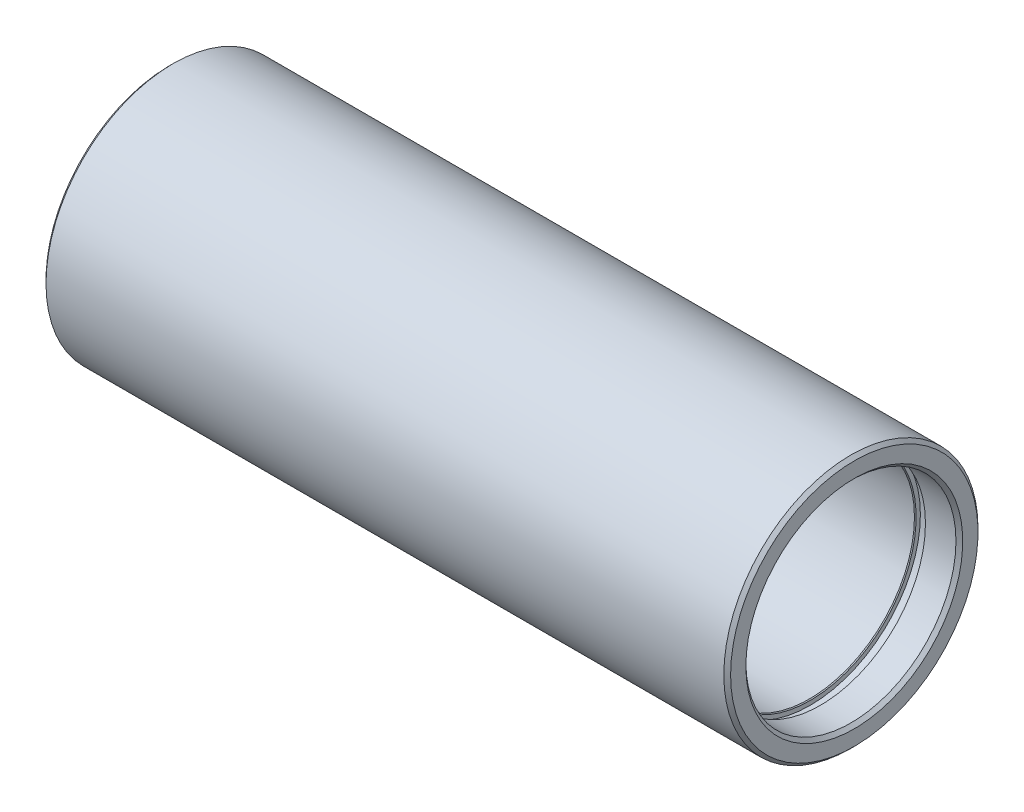
SolidWorks part; units mm, degrees
ref_plane "前视基准面" through (0, 0, 0) normal (0, 0, 1) x (1, 0, 0)
ref_plane "上视基准面" through (0, 0, 0) normal (0, 1, 0) x (1, 0, 0)
ref_plane "右视基准面" through (0, 0, 0) normal (1, 0, 0) x (0, 0, -1)
sketch "草图1" plane through (0, 0, 0) normal (0, 0, 1) x (1, 0, 0)
  line L0 (0, 0) -> (96.9258, 0) construction
  line L1 (-4.1244, 31) -> (5.8756, 31)
  line L2 (5.8756, 31) -> (5.8756, 32.5)
  line L3 (5.8756, 32.5) -> (8.8756, 32.5)
  line L4 (8.8756, 32.5) -> (8.8756, 31)
  line L5 (8.8756, 31) -> (184.8756, 31)
  line L6 (187.8756, 31) -> (187.8756, 32.5)
  line L7 (187.8756, 32.5) -> (184.8756, 32.5)
  line L8 (184.8756, 32.5) -> (184.8756, 31)
  line L9 (187.8756, 31) -> (197.8756, 31)
  line L10 (-4.1244, 31) -> (-4.1244, 37.5)
  line L11 (-4.1244, 37.5) -> (197.8756, 37.5)
  line L12 (197.8756, 37.5) -> (197.8756, 31)
  dimension "D1" = 31
  dimension "D2" = 202
  dimension "D3" = 10
  dimension "D4" = 3
  dimension "D5" = 1.5
  dimension "D6" = 10
  dimension "D7" = 3
  dimension "D8" = 1.5
  dimension "D9" = 6.5
revolve "旋转1" add sketch "草图1" angle 360 about L0
cosmetic thread "装饰螺纹线1" parameters "D2"=65.71
cosmetic thread "装饰螺纹线2" parameters "D2"=65.71
chamfer "倒角1" distance 1 angle 45 4 edges at (-4.1244, 0, 37.5) (-4.1244, 0, 31) (197.8756, 0, 37.5) (197.8756, 0, 31)
chamfer "倒角2" distance 0.25 angle 45 2 edges at (184.8756, 0, 31) (8.8756, 0, 31)
